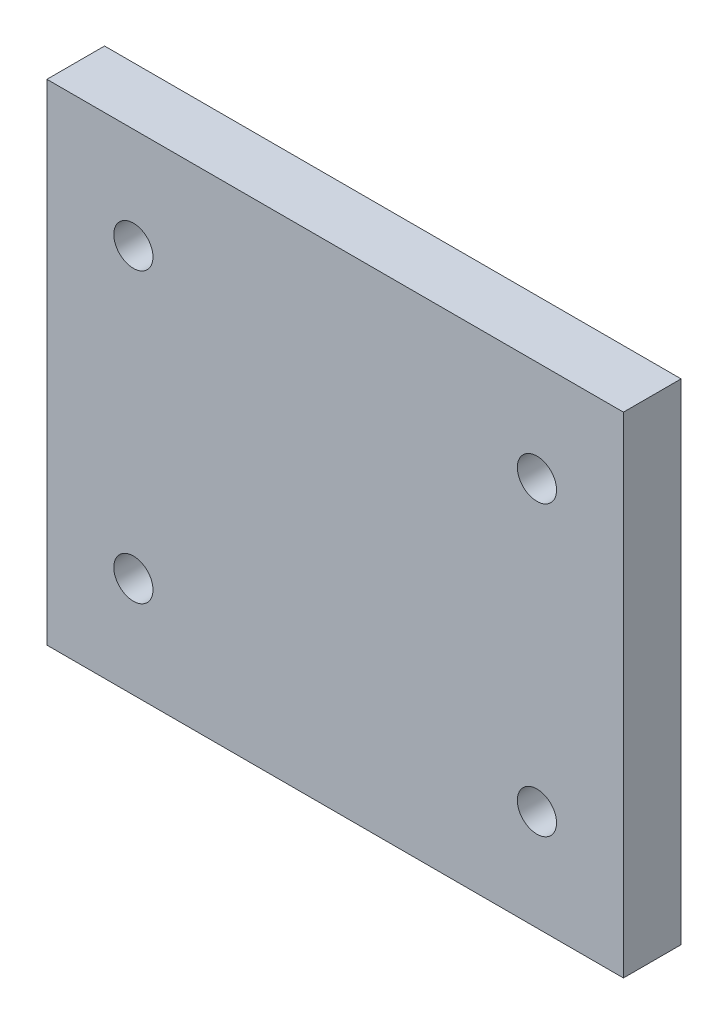
from build123d import *

# Parameters (mm, degrees)
SKETCH1_W             = 100
SKETCH1_H             = 85
BOSS_EXTRUDE1_DEPTH   = 10
M8_TAPPED_HOLE1_D     = 6.8
M8_TAPPED_HOLE1_DEPTH = 19.75
M8_TAPPED_HOLE1_TIP   = 2.042926105


with BuildPart() as part:
    # Sketch1 → Boss-Extrude1 (new body)
    with BuildSketch(Plane.XY):
        Rectangle(SKETCH1_W, SKETCH1_H)
    extrude(amount=BOSS_EXTRUDE1_DEPTH)

    # M8 Tapped Hole1
    with Locations(Plane.XY.offset(10)):
        with Locations((-35, 25), (35, 25), (35, -25), (-35, -25)):
            Hole(M8_TAPPED_HOLE1_D / 2, depth=M8_TAPPED_HOLE1_DEPTH)
            with Locations((0, 0, -(M8_TAPPED_HOLE1_DEPTH + M8_TAPPED_HOLE1_TIP / 2))):  # 118° drill point
                Cone(0, M8_TAPPED_HOLE1_D / 2, M8_TAPPED_HOLE1_TIP, mode=Mode.SUBTRACT)


solid = part.part
